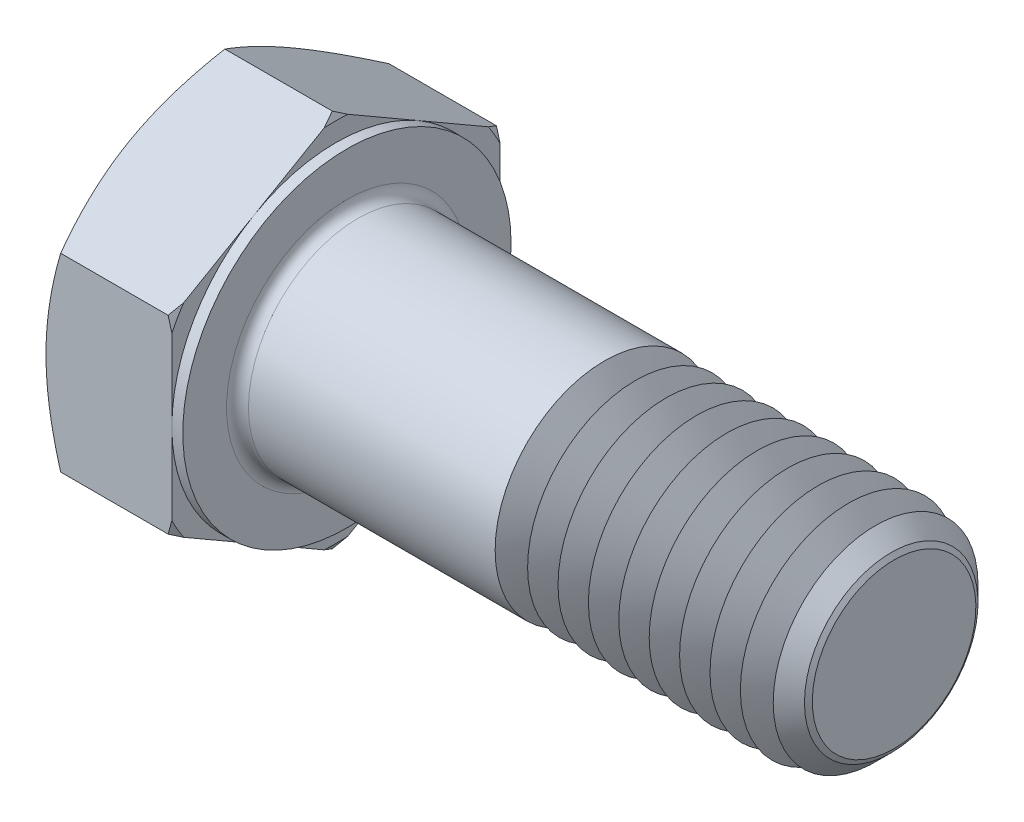
SolidWorks part; units mm, degrees
extrude "基体-拉伸" add sketch "草图1" along normal blind 7.5
sketch "草图1" plane through (0, 0, 0) normal (1, 0, 0) x (0, 0, -1)
  line L0 (9, 5.1962) -> (9, -5.1962)
  line L1 (-9, 5.1962) -> (-9, -5.1962)
  line L2 (9, -5.1962) -> (0, -10.3923)
  line L3 (0, -10.3923) -> (-9, -5.1962)
  line L4 (9, 5.1962) -> (0, 10.3923)
  line L5 (0, 10.3923) -> (-9, 5.1962)
revolve "切除-旋转1" cut sketch "草图3" angle 360 about L6
sketch "草图3" plane through (0, 0, 0) normal (0, 0, 1) x (1, 0, 0)
  line L0 (0, 9) -> (3.6906, 15.3923)
  line L1 (0, 10.3923) -> (0, 5.1962) construction
  line L2 (3.6906, 15.3923) -> (3.6906, 20.3923)
  line L3 (3.6906, 20.3923) -> (-10, 20.3923)
  line L4 (-10, 20.3923) -> (-10, 9)
  line L5 (-10, 9) -> (0, 9)
  line L6 (0, 0) -> (99.06, 0) construction
  line L7 (7.5, 10.3923) -> (0, 10.3923) construction
material "5.6级"
ref_plane "前视" through (0, 0, 0) normal (0, 0, 1) x (1, 0, 0)
ref_plane "上视" through (0, 0, 0) normal (0, 1, 0) x (1, 0, 0)
ref_plane "右视" through (0, 0, 0) normal (1, 0, 0) x (0, 0, -1)
sketch "草图2" plane through (0, 0, 0) normal (0, 0, 1) x (1, 0, 0)
  line L0 (0, 5.1962) -> (0, -5.1962) construction
  line L1 (0, 0) -> (37.5, 0)
  line L2 (0, 0) -> (0, 6)
  line L3 (0, 6) -> (7.7917, 6)
  line L4 (37.5, 0) -> (37.5, 4.4845)
  line L5 (7.5, 10.3923) -> (7.5, 5.1962) construction
  line L7 (0, 0) -> (96.52, 0) construction
  line L8 (37.5, -4.4845) -> (7.7917, -6) construction
  line L9 (0, -6) -> (7.7917, -6) construction
  line L10 (9.25, 15.24) -> (9.25, -1.27) construction
  line L11 (22.5, 15.24) -> (22.5, -1.27) construction
  line L12 (7.5, 5.1962) -> (7.5, -5.1962) construction
  line L13 (7.7917, 6) -> (37.5, 6)
  line L14 (37.5, 6) -> (37.5, 4.4845)
revolve "凸台-旋转1" add sketch "草图2" angle 360 about L7
cosmetic thread "螺旋线1" parameters "Thread_length"=15, "Thread_minor"=8.969
sketch "草图5" plane through (0, 0, 0) normal (0, 0, 1) x (1, 0, 0)
  line L0 (7.5, 9) -> (3.8094, 15.3923)
  line L1 (7.5, 10.3923) -> (7.5, 5.1962) construction
  line L2 (3.8094, 15.3923) -> (3.8094, 20.3923)
  line L3 (3.8094, 20.3923) -> (13.8094, 20.3923)
  line L4 (13.8094, 20.3923) -> (13.8094, 9)
  line L5 (13.8094, 9) -> (7.5, 9)
  line L7 (7.5, 10.3923) -> (0.8038, 10.3923) construction
  line L8 (0, 0) -> (99.06, 0) construction
  line L9 (0, 0) -> (99.06, 0) construction
revolve "切除-旋转2" cut sketch "草图5" angle 360 about L8
sketch "草图4" plane through (0, 0, 0) normal (0, 0, 1) x (1, 0, 0)
  line L1 (7.5, 10.3923) -> (7.5, 5.1962) construction
  line L2 (7.5, 9) -> (6.9, 9)
  line L3 (7.5, 9) -> (7.5, 20.3923)
  line L4 (7.5, 20.3923) -> (6.9, 20.3923)
  line L5 (0, 0) -> (95.25, 0) construction
  line L6 (0, 0) -> (96.52, 0) construction
  line L7 (6.9, 9) -> (6.9, 20.3923)
  line L8 (6.6962, 10.3923) -> (0.8038, 10.3923) construction
revolve "切除-旋转3" cut sketch "草图4" angle 360 about L5
chamfer "倒角" distance 1.4 angle 45 1 edges at (37.5, 0, 6)
fillet "圆角" radius 0.6 1 edges at (7.5, 0, -6)
sketch "草图6" plane through (0, 0, 0) normal (0, 0, 1) x (1, 0, 0)
  line L0 (22.5, -4.4845) -> (21.625, -6)
  line L1 (22.5, -4.4845) -> (23.375, -6)
  line L2 (23.375, -6) -> (23.375, -7.5)
  line L3 (-3.175, 0) -> (5.1513, 0) construction
  line L5 (23.375, -7.5) -> (21.625, -7.5)
  line L6 (21.625, -7.5) -> (21.625, -6)
revolve "切除-旋转4" cut sketch "草图6" angle 360 about L3
pattern_linear "阵列(线性)1" count 10 spacing 1.6667 along (1, 0, 0) of "切除-旋转4"
equation "\"D3@草图1\" = \"s@草图1\" / 2"
equation "\"D4@草图1\" = \"D3@草图1\""
equation "\"D5@草图1\" = \"D4@草图1\""
equation "\"Thread_minor@螺旋线1\" = \"Minor_dia@草图2\""
equation "\"D1@草图3\" = \"s@草图1\" / 2"
equation "\"D1@草图5\" = \"s@草图1\" / 2"
equation "\"Head_ch_ang@草图5\" = \"Head_ch_ang@草图3\""
equation "\"D1@草图4\" = \"s@草图1\""
equation "\"Thread_length@螺旋线1\" = ((sgn( (\"l@草图2\" - \"p@草图2\" ) - \"h@草图2\" )-1)*( (\"l@草图2\" - \"p@草图2\" ) - \"h@草图2\" ))/-2+ \"h@草图2\""
equation "\"Thread_minor@草图6\" = \"Minor_dia@草图2\""
equation "\"Diameter@草图6\" = \"m@草图2\""
equation "\"Overcut@草图6\" = \"m@草图2\" * 1.25"
equation "\"Start@草图6\" = \"k@基体-拉伸\" + \"l@草图2\" - \"Thread_length@螺旋线1\"  '---Non-countersunk---"
equation "\"Num_threads@阵列(线性)1\" = int( \"Thread_length@螺旋线1\" / \"p@草图2\" + 0.999 )  + 1"
equation "\"Advance@阵列(线性)1\" = \"Thread_length@螺旋线1\" /  (\"Num_threads@阵列(线性)1\" - 1) 'relax it"
equation "\"Num_threads@阵列(线性)1\" = \"Num_threads@阵列(线性)1\" - sgn( \"Num_threads@阵列(线性)1\" - 1) '---chamfered tips only---"
equation "\"Minor_dia@草图2\" = \"m@草图2\"-\"p@草图2\" * 1.732"
equation "\"D1@倒角\" = \"p@草图2\"*0.8"
